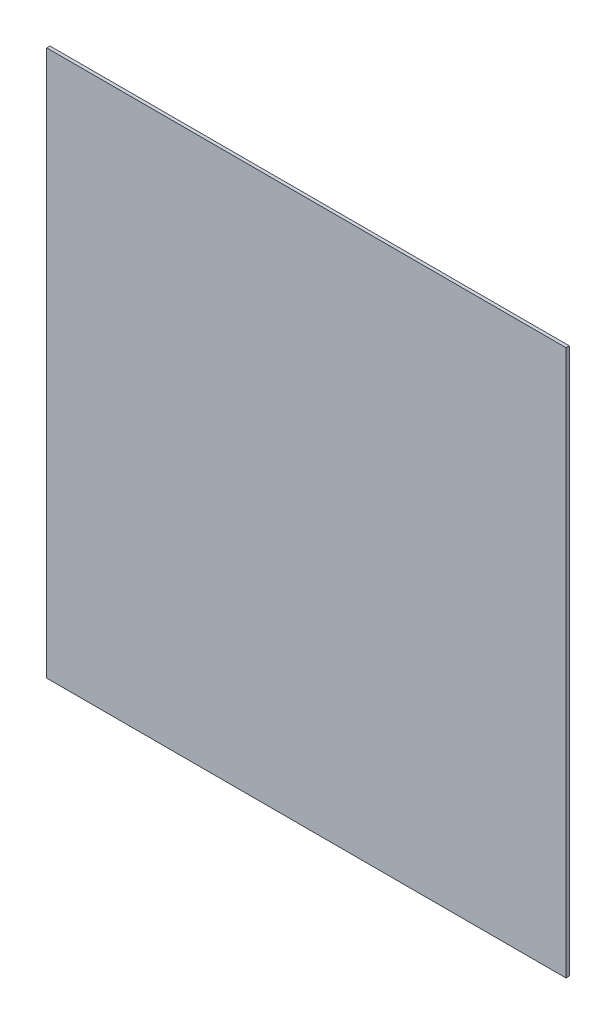
SolidWorks part; units mm, degrees
material "PMMA(有机玻璃)"
ref_plane "前视" through (0, 0, 0) normal (0, 0, 1) x (1, 0, 0)
ref_plane "上视" through (0, 0, 0) normal (0, 1, 0) x (1, 0, 0)
ref_plane "右视" through (0, 0, 0) normal (1, 0, 0) x (0, 0, -1)
sketch "草图1" plane through (0, 0, 0) normal (0, 0, 1) x (1, 0, 0)
  line L1 (-400.5, 421) -> (400.5, 421)
  line L2 (-400.5, 421) -> (-400.5, -421)
  line L3 (-400.5, -421) -> (400.5, -421)
  line L4 (400.5, 421) -> (400.5, -421)
  line L5 (-400.5, 421) -> (400.5, -421) construction
  line L6 (-400.5, -421) -> (400.5, 421) construction
  point P0 (0, 0)
  dimension "D1" = 842
  dimension "D2" = 801
extrude "凸台-拉伸1" add sketch "草图1" along normal blind 5
hole_wizard "M5 间隙孔1" positions "草图3" profile "草图2" hole size "M5" standard "GB"
sketch "草图3" plane through (0, 0, 5) normal (0, 0, 1) x (1, 0, 0)
  line L0 (-427.5, 273) -> (-427.5, -273) construction
  line L1 (-427.5, -273) -> (427.5, -273) construction
  line L2 (0, 273) -> (0, -273) construction
  line L3 (427.5, 273) -> (-427.5, 273) construction
  line L5 (-427.5, 0) -> (427.5, 0) construction
  line L6 (427.5, -273) -> (427.5, 273) construction
  point P0 (-375, -261)
  point P46 (415.5, 250)
  point P48 (-415.5, 250)
  point P58 (-125, -261)
  point P59 (125, -261)
  point P61 (-125, 261)
  point P62 (125, 261)
  point P64 (-375, 261)
  point P88 (375, -261)
  point P89 (375, 261)
  point P108 (415.5, 0)
  point P109 (-415.5, 0)
  point P110 (415.5, -250)
  point P111 (-415.5, -250)
  dimension "D1" = 12
  dimension "D2" = 12
  dimension "D5" = 3
  dimension "D3" = 12
  dimension "D6" = 4
  dimension "D4" = 2
sketch "草图2" plane through (-375, -261, 5) normal (1, 0, 0) x (0, -1, 0)
  line L0 (0, 0) -> (0, 5)
  line L1 (0, 5) -> (2.75, 5)
  line L2 (2.75, 5) -> (2.75, 0)
  line L5 (2.75, 0) -> (0, 0)
  line L11 (0, -6.35) -> (0, 107.95) construction
  dimension "通孔孔直径" = 5.5
  dimension "通孔孔深度" = 5
